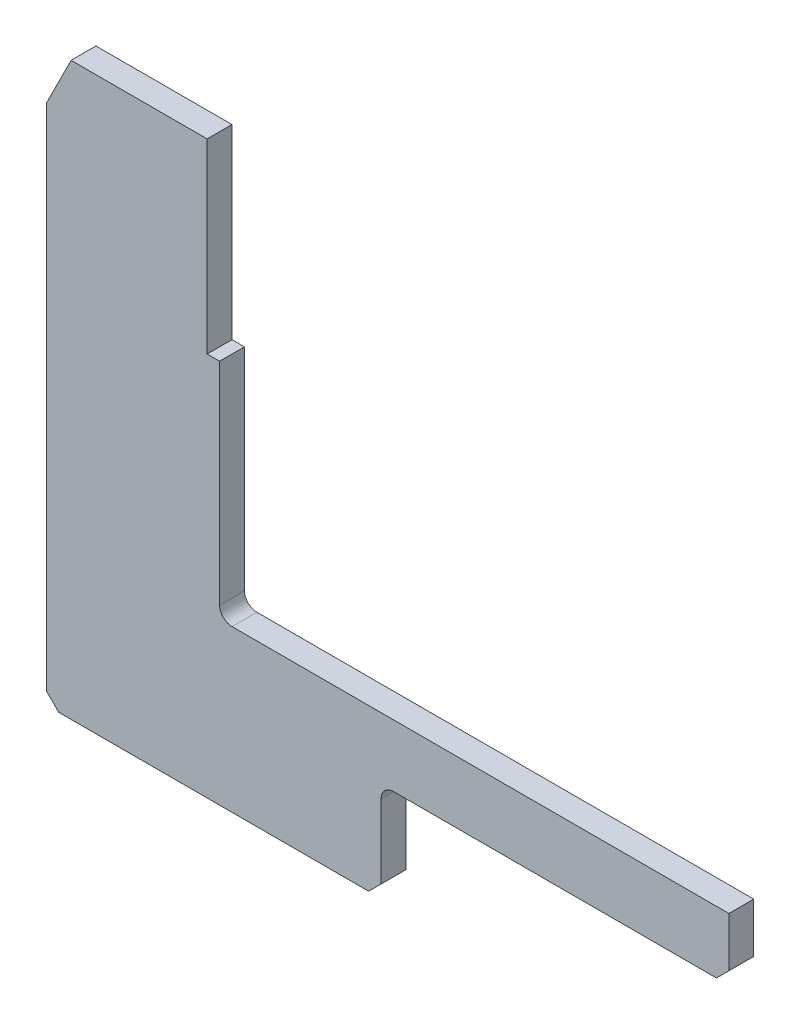
SolidWorks part; units mm, degrees
ref_plane "Front Plane" through (0, 0, 0) normal (0, 0, 1) x (1, 0, 0)
ref_plane "Top Plane" through (0, 0, 0) normal (0, 1, 0) x (1, 0, 0)
ref_plane "Right Plane" through (0, 0, 0) normal (1, 0, 0) x (0, 0, -1)
sketch "Sketch1" plane through (0, 0, 0) normal (0, 0, 1) x (1, 0, 0)
  line L0 (-572.5787, 758.2468) -> (-572.5787, -80.7532)
  line L1 (-572.5787, -80.7532) -> (-33.5787, -80.7532)
  line L2 (-33.5787, -80.7532) -> (-33.5787, 78.2468)
  line L3 (-33.5787, 78.2468) -> (526.4213, 78.2468)
  line L4 (526.4213, 78.2468) -> (526.4213, 178.2468)
  line L5 (526.4213, 178.2468) -> (-293.5787, 178.2468)
  line L6 (-293.5787, 178.2468) -> (-293.5787, 538.2468)
  line L7 (-293.5787, 538.2468) -> (-313.5787, 538.2468)
  line L8 (-313.5787, 538.2468) -> (-313.5787, 838.2468)
  line L9 (-313.5787, 838.2468) -> (-532.5787, 838.2468)
  line L12 (-572.5787, 758.2468) -> (-532.5787, 838.2468)
extrude "Boss-Extrude1" add sketch "Sketch1" along normal blind 40
chamfer "Chamfer1" distance 20 angle 45 3 edges at (-572.5787, -80.7532, 20) (526.4213, 78.2468, 20) (-33.5787, -80.7532, 20)
fillet "Fillet1" radius 20 2 edges at (-33.5787, 78.2468, 20) (-293.5787, 178.2468, 20)
